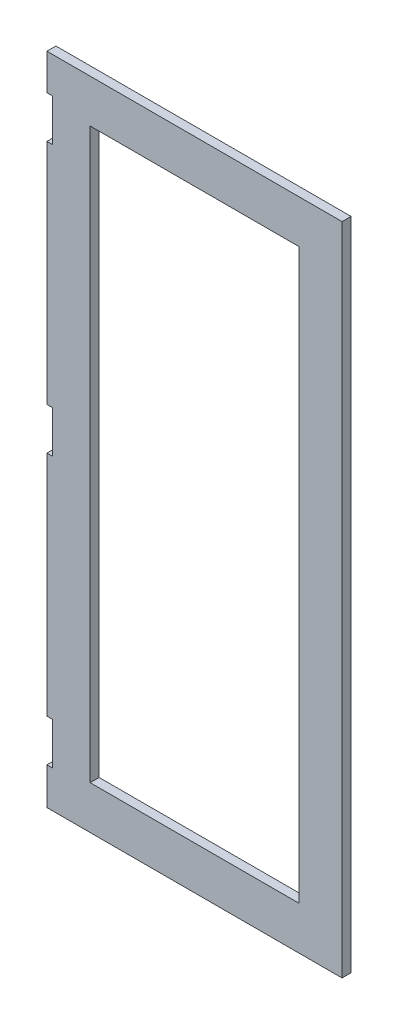
SolidWorks part; units mm, degrees
ref_plane "前视基准面" through (0, 0, 0) normal (0, 0, 1) x (1, 0, 0)
ref_plane "上视基准面" through (0, 0, 0) normal (0, 1, 0) x (1, 0, 0)
ref_plane "右视基准面" through (0, 0, 0) normal (1, 0, 0) x (0, 0, -1)
sketch "草图1" plane through (0, 0, 0) normal (0, 0, 1) x (1, 0, 0)
  line L1 (-410, 910) -> (410, 910)
  line L2 (-410, 910) -> (-410, -910)
  line L3 (-410, -910) -> (410, -910)
  line L4 (410, 910) -> (410, -910)
  line L5 (-410, 910) -> (410, -910) construction
  line L6 (-410, -910) -> (410, 910) construction
  point P0 (0, 0)
  dimension "D1" = 820
  dimension "D2" = 1820
extrude "凸台-拉伸1" add sketch "草图1" along normal blind 25
sketch "草图2" plane through (0, 0, 25) normal (0, 0, 1) x (1, 0, 0)
  line L0 (410, 910) -> (-410, 910) construction
  line L1 (-290, -790) -> (290, -790)
  line L2 (-290, -790) -> (-290, 790)
  line L3 (-290, 790) -> (290, 790)
  line L4 (290, -790) -> (290, 790)
  line L5 (-290, -790) -> (290, 790) construction
  line L6 (-290, 790) -> (290, -790) construction
  line L7 (410, -910) -> (410, 910) construction
  point P0 (0, 0)
  dimension "D1" = 120
  dimension "D2" = 120
extrude "切除-拉伸1" cut sketch "草图2" against normal through all
sketch "草图3" plane through (0, 0, 25) normal (0, 0, 1) x (1, 0, 0)
  line L0 (-410, 910) -> (-410, -910) construction
  line L1 (-410, -690) -> (-395, -690)
  line L2 (-410, -690) -> (-410, -807)
  line L3 (-410, -807) -> (-395, -807)
  line L4 (-395, -690) -> (-395, -807)
  line L5 (-410, -910) -> (410, -910) construction
  line L6 (-410, -57) -> (-395, -57)
  line L7 (-395, 60) -> (-395, -57)
  line L8 (-410, 60) -> (-410, -57)
  line L9 (-410, 60) -> (-395, 60)
  line L10 (-410, 693) -> (-395, 693)
  line L11 (-395, 810) -> (-395, 693)
  line L12 (-410, 810) -> (-410, 693)
  line L13 (-410, 810) -> (-395, 810)
  dimension "D1" = 103
  dimension "D2" = 117
  dimension "D3" = 15
  dimension "D4" = 3
extrude "切除-拉伸2" cut sketch "草图3" against normal through all
